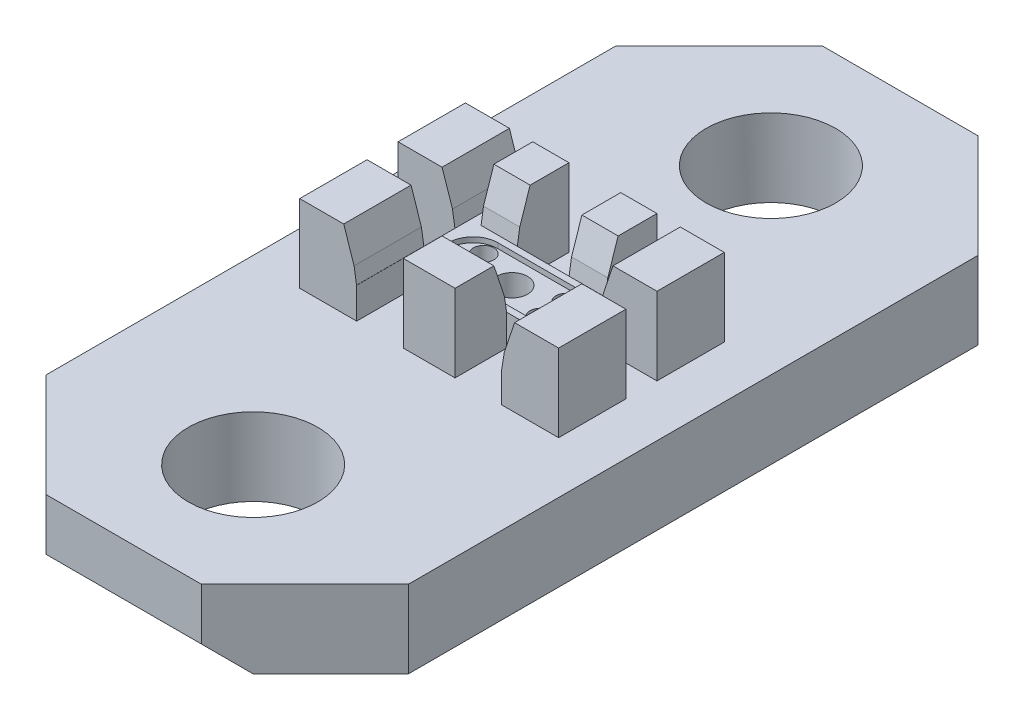
SolidWorks part; units mm, degrees
ref_plane "Front Plane" through (0, 0, 0) normal (0, 0, 1) x (1, 0, 0)
ref_plane "Top Plane" through (0, 0, 0) normal (0, 1, 0) x (1, 0, 0)
ref_plane "Right Plane" through (0, 0, 0) normal (1, 0, 0) x (0, 0, -1)
sketch "Sketch1" plane through (0, 0, 0) normal (0, 1, 0) x (1, 0, 0)
  line L1 (-3.5, 7.5) -> (3.5, 7.5)
  line L2 (-3.5, 7.5) -> (-3.5, -7.5)
  line L3 (-3.5, -7.5) -> (3.5, -7.5)
  line L4 (3.5, 7.5) -> (3.5, -7.5)
  line L5 (-3.5, 7.5) -> (3.5, -7.5) construction
  line L6 (-3.5, -7.5) -> (3.5, 7.5) construction
  point P0 (0, 0)
  dimension "D1" = 7
  dimension "D2" = 15
extrude "Boss-Extrude1" add sketch "Sketch1" along normal blind 1.5
sketch "Sketch2" plane through (0, 1.5, 0) normal (0, 1, 0) x (1, 0, 0)
  line L0 (3.5, 7.5) -> (-3.5, 7.5) construction
  line L1 (0, 0) -> (0, 50000) construction
  line L2 (-2.5, -1.6) -> (-2.5, 1.6)
  line L4 (2.5, -1.6) -> (2.5, 1.6)
  line L5 (-1.6207, -4.0517) -> (3, 7.5) construction
  line L6 (-3, 3.5) -> (3, -3.5) construction
  line L8 (-2.5, 1.6) -> (2.5, 1.6)
  line L9 (0, 0) -> (50000, 0) construction
  line L10 (-2.5, -1.6) -> (2.5, -1.6)
  point P0 (0, 0)
  dimension "D1" = 5
  dimension "D2" = 3.2
extrude "Boss-Extrude2" add sketch "Sketch2" along normal blind 1.5
sketch "Sketch3" plane through (0, 3, 0) normal (0, 1, 0) x (1, 0, 0)
  line L1 (-1.45, 0.65) -> (1.45, 0.65)
  line L2 (-1.45, 0.65) -> (-1.45, -0.65)
  line L3 (-1.45, -0.65) -> (1.45, -0.65)
  line L4 (1.45, 0.65) -> (1.45, -0.65)
  line L5 (-1.45, 0.65) -> (1.45, -0.65) construction
  line L6 (-1.45, -0.65) -> (1.45, 0.65) construction
  point P0 (0, 0)
  dimension "D1" = 2.9
  dimension "D2" = 1.3
extrude "Cut-Extrude1" cut sketch "Sketch3" against normal blind 0.9
sketch "Sketch4" plane through (0, 0, 0) normal (0, -1, 0) x (1, 0, 0)
  line L0 (0.1934, 0) -> (50000.1934, 0) construction
  line L1 (0, 0) -> (0, -50000) construction
  line L2 (-0.75, 0) -> (0.75, 0) construction
  line L3 (-0.75, 0.6) -> (0.75, 0.6)
  line L4 (-0.75, -0.6) -> (0.75, -0.6)
  line L5 (3.5, 7.5) -> (3.5, -7.5) construction
  line L6 (-3.5, -7.5) -> (-3.5, 7.5) construction
  line L7 (-3.5, 7.5) -> (3.5, 7.5) construction
  line L8 (3.5, -7.5) -> (-3.5, -7.5) construction
  arc A1 (-0.75, 0.6) -> (-0.75, -0.6) centre (-0.75, 0) ccw
  arc A2 (0.75, -0.6) -> (0.75, 0.6) centre (0.75, 0) ccw
  point P8 (0, 0)
  dimension "D1" = 1.5
  dimension "D2" = 1.2
extrude "Cut-Extrude2" cut sketch "Sketch4" against normal blind 1
chamfer "Chamfer1" distance 0.2 distance2 0.6 2 edges at (0, 3, 0.65) (0, 3, -0.65)
chamfer "Chamfer2" distance 0.2 distance2 0.6 2 edges at (-1.45, 3, 0) (1.45, 3, 0)
chamfer "Chamfer3" distance 2 angle 45 4 edges at (3.5, 0.75, -7.5) (3.5, 0.75, 7.5) (-3.5, 0.75, -7.5) (-3.5, 0.75, 7.5)
sketch "Sketch8" plane through (0, 1.5, 0) normal (0, 1, 0) x (1, 0, 0)
  line L0 (0, 0) -> (0, 50000) construction
  line L1 (0, 0) -> (-6.9373, 0) construction
  circle A0 centre (0, -5) radius 1.25
  circle A1 centre (0, 5) radius 1.25
  dimension "D1" = 10
  dimension "D2" = 2.5
extrude "Cut-Extrude6" cut sketch "Sketch8" against normal blind 2
sketch "Sketch9" plane through (0, 2.1, 0) normal (0, 1, 0) x (1, 0, 0)
  line L0 (0, 0) -> (50000, 0) construction
  line L1 (0, 0) -> (0, 50000) construction
  circle A0 centre (-0.8, 0.25) radius 0.2
  circle A1 centre (0.8, 0.25) radius 0.2
  circle A2 centre (0.8, -0.25) radius 0.2
  circle A3 centre (-0.8, -0.25) radius 0.2
  dimension "D1" = 0.5
  dimension "D2" = 0.4
  dimension "D3" = 1.6
extrude "Cut-Extrude7" cut sketch "Sketch9" against normal through all
sketch "Sketch10" plane through (0, 2.1, 0) normal (0, 1, 0) x (1, 0, 0)
  line L0 (-0.75, 0) -> (0.75, 0) construction
  line L1 (-0.75, 0.475) -> (0.75, 0.475)
  line L2 (-0.75, -0.475) -> (0.75, -0.475)
  arc A0 (-0.75, 0.475) -> (-0.75, -0.475) centre (-0.75, 0) ccw
  arc A1 (0.75, -0.475) -> (0.75, 0.475) centre (0.75, 0) ccw
  point P2 (0, 0)
  dimension "D1" = 1.5
  dimension "D2" = 0.95
extrude "Cut-Extrude8" cut sketch "Sketch10" against normal blind 0.1
sketch "Sketch12" plane through (0, 0, 0) normal (1, 0, 0) x (0, 0, -1)
  line L0 (-0.65, 2.4) -> (-0.6025, 2.1)
  line L1 (-0.65, 2.1) -> (0.65, 2.1) construction
  line L2 (-0.6025, 2.1) -> (-0.65, 2.1)
  line L3 (-0.65, 2.1) -> (-0.65, 2.4)
  line L4 (0, 0) -> (0, 50000) construction
  line L5 (0.65, 2.1) -> (0.65, 2.4)
  line L6 (0.6025, 2.1) -> (0.65, 2.1)
  line L7 (0.65, 2.4) -> (0.6025, 2.1)
  dimension "D1" = 18
extrude "Boss-Extrude3" add sketch "Sketch12" along normal mid plane 3.1
sketch "Sketch15" plane through (0, 0, 0) normal (0, 0, 1) x (1, 0, 0)
  line L0 (-1.45, 2.4) -> (-1.4025, 2.1)
  line L1 (1.45, 2.1) -> (-1.45, 2.1) construction
  line L2 (-1.4025, 2.1) -> (-1.45, 2.1)
  line L3 (-1.45, 2.1) -> (-1.45, 2.4)
  line L4 (0, 1.5) -> (0, 50001.5) construction
  line L5 (-1.5, 1.5) -> (1.5, 1.5) construction
  line L6 (1.45, 2.1) -> (1.45, 2.4)
  line L7 (1.4025, 2.1) -> (1.45, 2.1)
  line L8 (1.45, 2.4) -> (1.4025, 2.1)
  point P11 (0, 1.5)
  dimension "D1" = 18
extrude "Boss-Extrude4" add sketch "Sketch15" along normal mid plane 1.3
sketch "Sketch5" plane through (0, 3, 0) normal (0, 1, 0) x (1, 0, 0)
  line L0 (0, 0) -> (0, 50000) construction
  line L1 (1.5, 7.5) -> (-1.5, 7.5) construction
  line L3 (-0.5, 6.5) -> (0.5, 6.5)
  line L4 (-0.5, 6.5) -> (-0.5, 0.6025)
  line L5 (1.4025, 0.6025) -> (-1.4025, 0.6025) construction
  line L6 (0.5, 6.5) -> (0.5, 0.6025)
  line L7 (1.5, 7.5) -> (-1.5, 7.5) construction
  line L9 (0.5, 0.6025) -> (-0.5, 0.6025)
  point P5 (0, 7.5)
  point P6 (0, 1.3773)
  dimension "D1" = 1
  dimension "D2" = 1
extrude "Cut-Extrude3" cut sketch "Sketch5" against normal up to surface (1.5 mm away) up to face at (0, 1.5, -6.25)
sketch "Sketch6" plane through (0, 3, 0) normal (0, 1, 0) x (1, 0, 0)
  line L0 (0, 0) -> (0, 50000) construction
  line L1 (0, 0) -> (-50000, 0) construction
  line L3 (-2.5, 0.3) -> (-1.4025, 0.3)
  line L4 (-2.5, 0.3) -> (-2.5, -0.3)
  line L5 (-2.5, -0.3) -> (-1.4025, -0.3)
  line L6 (-1.4025, -0.6025) -> (-1.4025, 0.6025) construction
  line L7 (1.4025, -0.3) -> (1.4025, 0.3)
  line L8 (2.5, -0.3) -> (1.4025, -0.3)
  line L9 (-2.5, 1.6) -> (-2.5, -1.6) construction
  line L10 (2.5, 0.3) -> (2.5, -0.3)
  line L11 (2.5, 0.3) -> (1.4025, 0.3)
  line L16 (-1.4025, -0.3) -> (-1.4025, 0.3)
  point P5 (-1.975, 0)
  point P14 (1.975, 0)
  dimension "D1" = 0.6
extrude "Cut-Extrude4" cut sketch "Sketch6" against normal up to surface (1.5 mm away) up to face at (0, 1.5, -6.25)
sketch "Sketch7" plane through (0, 3, 0) normal (0, 1, 0) x (1, 0, 0)
  line L0 (0, 0) -> (0, -50000) construction
  line L1 (0, 0) -> (-50000, 0) construction
  line L4 (-1.4, -0.6025) -> (-1.4, -1.6)
  line L5 (-1.4, -1.6) -> (-0.5, -1.6)
  line L6 (-0.5, -0.6025) -> (-0.5, -1.6)
  line L7 (-2.5, -1.6) -> (2.5, -1.6) construction
  line L8 (1.4025, -0.6025) -> (-1.4025, -0.6025) construction
  line L9 (-0.5, -0.6025) -> (-1.4, -0.6025)
  line L10 (0.95, -1.75) -> (0.95, 49998.25) construction
  line L11 (0.5, -0.6025) -> (1.4, -0.6025)
  line L12 (-0.95, -1.75) -> (-0.95, 49998.25) construction
  line L13 (0.95, -0.64) -> (0.95, -50000.64) construction
  line L14 (0.5, -0.6025) -> (0.5, -1.6)
  line L15 (1.4, -1.6) -> (0.5, -1.6)
  line L16 (1.4, -0.6025) -> (1.4, -1.6)
  point P19 (-0.95, -1.6)
  dimension "D1" = 1.9
  dimension "D2" = 0.9
  dimension "D3" = 0.95
extrude "Cut-Extrude5" cut sketch "Sketch7" against normal up to surface (1.5 mm away) up to face at (0, 1.5, -6.25)
chamfer "Chamfer5" distance 0.25 distance2 0.6 2 edges at (1.4, 3, 1.225) (-1.4, 3, 1.225)
sketch "Sketch16" plane through (0, 0, 1.6) normal (0, 0, 1) x (1, 0, 0)
  line L0 (-1.45, 2.4) -> (-1.65, 3) construction
  line L1 (-1.45, 2.4) -> (-1.4025, 2.1) construction
  line L3 (-1.4, 2.4) -> (-1.65, 3) construction
  line L4 (-1.45, 2.4) -> (-1.65, 3)
  line L5 (-1.45, 2.4) -> (-1.4025, 2.1)
  line L6 (-1.4025, 2.1) -> (-1.3203, 2.1)
  line L7 (-1.4, 2.4) -> (-1.65, 3)
  line L8 (0, 3) -> (0, -49997) construction
  line L9 (-0.5, 3) -> (0.5, 3) construction
  line L10 (1.3203, 2.4) -> (1.3203, 2.1)
  line L11 (1.4, 2.4) -> (1.3203, 2.4)
  line L12 (1.4, 2.4) -> (1.65, 3)
  line L13 (1.4025, 2.1) -> (1.3203, 2.1)
  line L14 (-1.4, 2.4) -> (-1.3203, 2.4)
  line L15 (-0.5, 2.4) -> (-1.45, 2.4) construction
  line L16 (-1.3203, 2.4) -> (-1.3203, 2.1)
  line L18 (1.45, 2.4) -> (1.4025, 2.1)
  line L19 (1.45, 2.4) -> (1.65, 3)
  point P8 (0, 3)
extrude "Cut-Extrude9" cut sketch "Sketch16" against normal blind 1.3
sketch "Sketch18" plane through (0, 0, 1.6) normal (0, 0, 1) x (1, 0, 0)
  line L0 (-1.4025, 2.1) -> (-1.2, 2.1)
  line L1 (-0.5, 2.1) -> (-1.4, 2.1) construction
  line L2 (-1.2, 2.1) -> (-1.2, 3.1667)
  line L3 (-1.2, 3.1667) -> (-1.7056, 3.1667)
  line L4 (-1.65, 3) -> (-1.45, 2.4) construction
  line L5 (-1.45, 2.4) -> (-1.4025, 2.1) construction
  line L6 (-1.7056, 3.1667) -> (-1.45, 2.4)
  line L7 (-1.45, 2.4) -> (-1.4025, 2.1)
  line L8 (-0.5, 3) -> (-0.5, 2.4) construction
  line L9 (0, 0) -> (0, 50000) construction
  line L10 (1.45, 2.4) -> (1.4025, 2.1)
  line L11 (1.7056, 3.1667) -> (1.45, 2.4)
  line L12 (1.2, 3.1667) -> (1.7056, 3.1667)
  line L13 (1.2, 2.1) -> (1.2, 3.1667)
  line L14 (1.4025, 2.1) -> (1.2, 2.1)
  dimension "D1" = 0.7
extrude "Cut-Extrude10" cut sketch "Sketch18" against normal blind 3.3
sketch "Sketch19" plane through (0, 1, 0) normal (0, -1, 0) x (1, 0, 0)
  circle A0 centre (0, 0) radius 0.3
  dimension "D1" = 0.6
extrude "Cut-Extrude11" cut sketch "Sketch19" against normal blind 10
chamfer "Chamfer6" distance 0.5 angle 45 3 edges at (-3.5, 0, 0) (0, 0, -7.5) (0, 0, 7.5)
